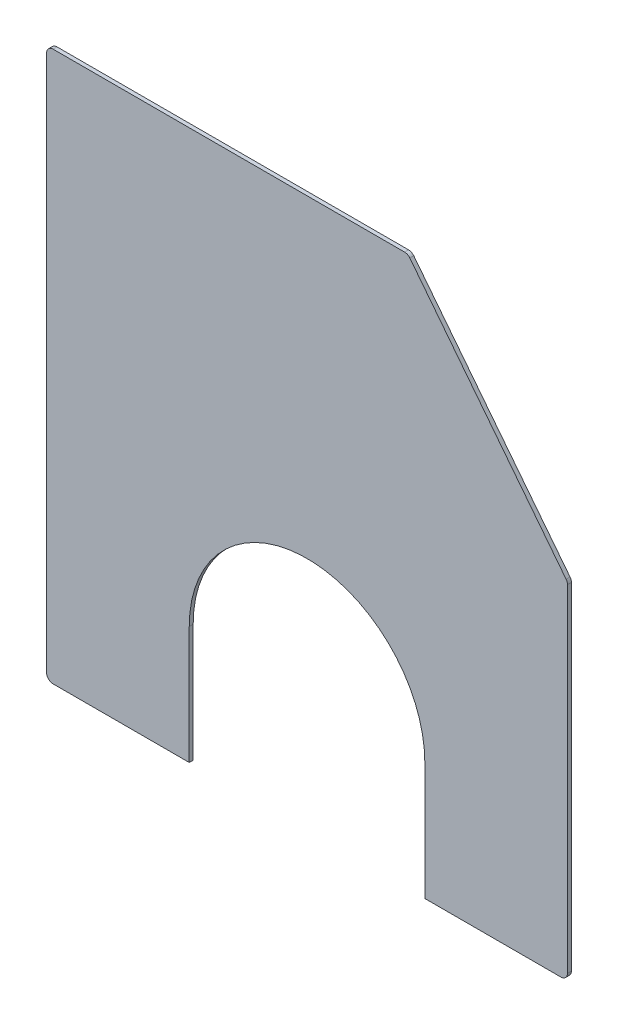
SolidWorks part; units mm, degrees
ref_plane "Front Plane" through (0, 0, 0) normal (0, 0, 1) x (1, 0, 0)
ref_plane "Top Plane" through (0, 0, 0) normal (0, 1, 0) x (1, 0, 0)
ref_plane "Right Plane" through (0, 0, 0) normal (1, 0, 0) x (0, 0, -1)
sketch "Sketch1" plane through (0, 0, 0) normal (0, 0, 1) x (1, 0, 0)
  line L0 (0, 5) -> (0, 415)
  line L1 (5, 420) -> (273.6027, 420)
  line L2 (277.5427, 418.0783) -> (396.9401, 265.2567)
  line L3 (398, 262.1784) -> (398, 5)
  line L4 (393, 0) -> (289, 0)
  line L5 (109, 90) -> (109, 0)
  line L6 (289, 90) -> (289, 0)
  line L7 (109, 0) -> (5, 0)
  arc A0 (289, 90) -> (109, 90) centre (199, 90) ccw
  arc A1 (0, 5) -> (5, 0) centre (5, 5) ccw
  arc A2 (398, 5) -> (393, 0) centre (393, 5) cw
  arc A3 (396.9401, 265.2567) -> (398, 262.1784) centre (393, 262.1784) cw
  arc A4 (273.6027, 420) -> (277.5427, 418.0783) centre (273.6027, 415) cw
  arc A5 (0, 415) -> (5, 420) centre (5, 415) cw
  point P13 (0, 0)
  point P16 (398, 0)
  point P19 (398, 263.9)
  point P24 (0, 420)
  dimension "D2" = 180
  dimension "D4" = 199
  dimension "D9" = 5
  dimension "D1" = 398
  dimension "D3" = 90
  dimension "D5" = 263.9
  dimension "D6" = 90
  dimension "D7" = 142
  dimension "D8" = 420
extrude "Boss-Extrude1" add sketch "Sketch1" along normal blind 3
